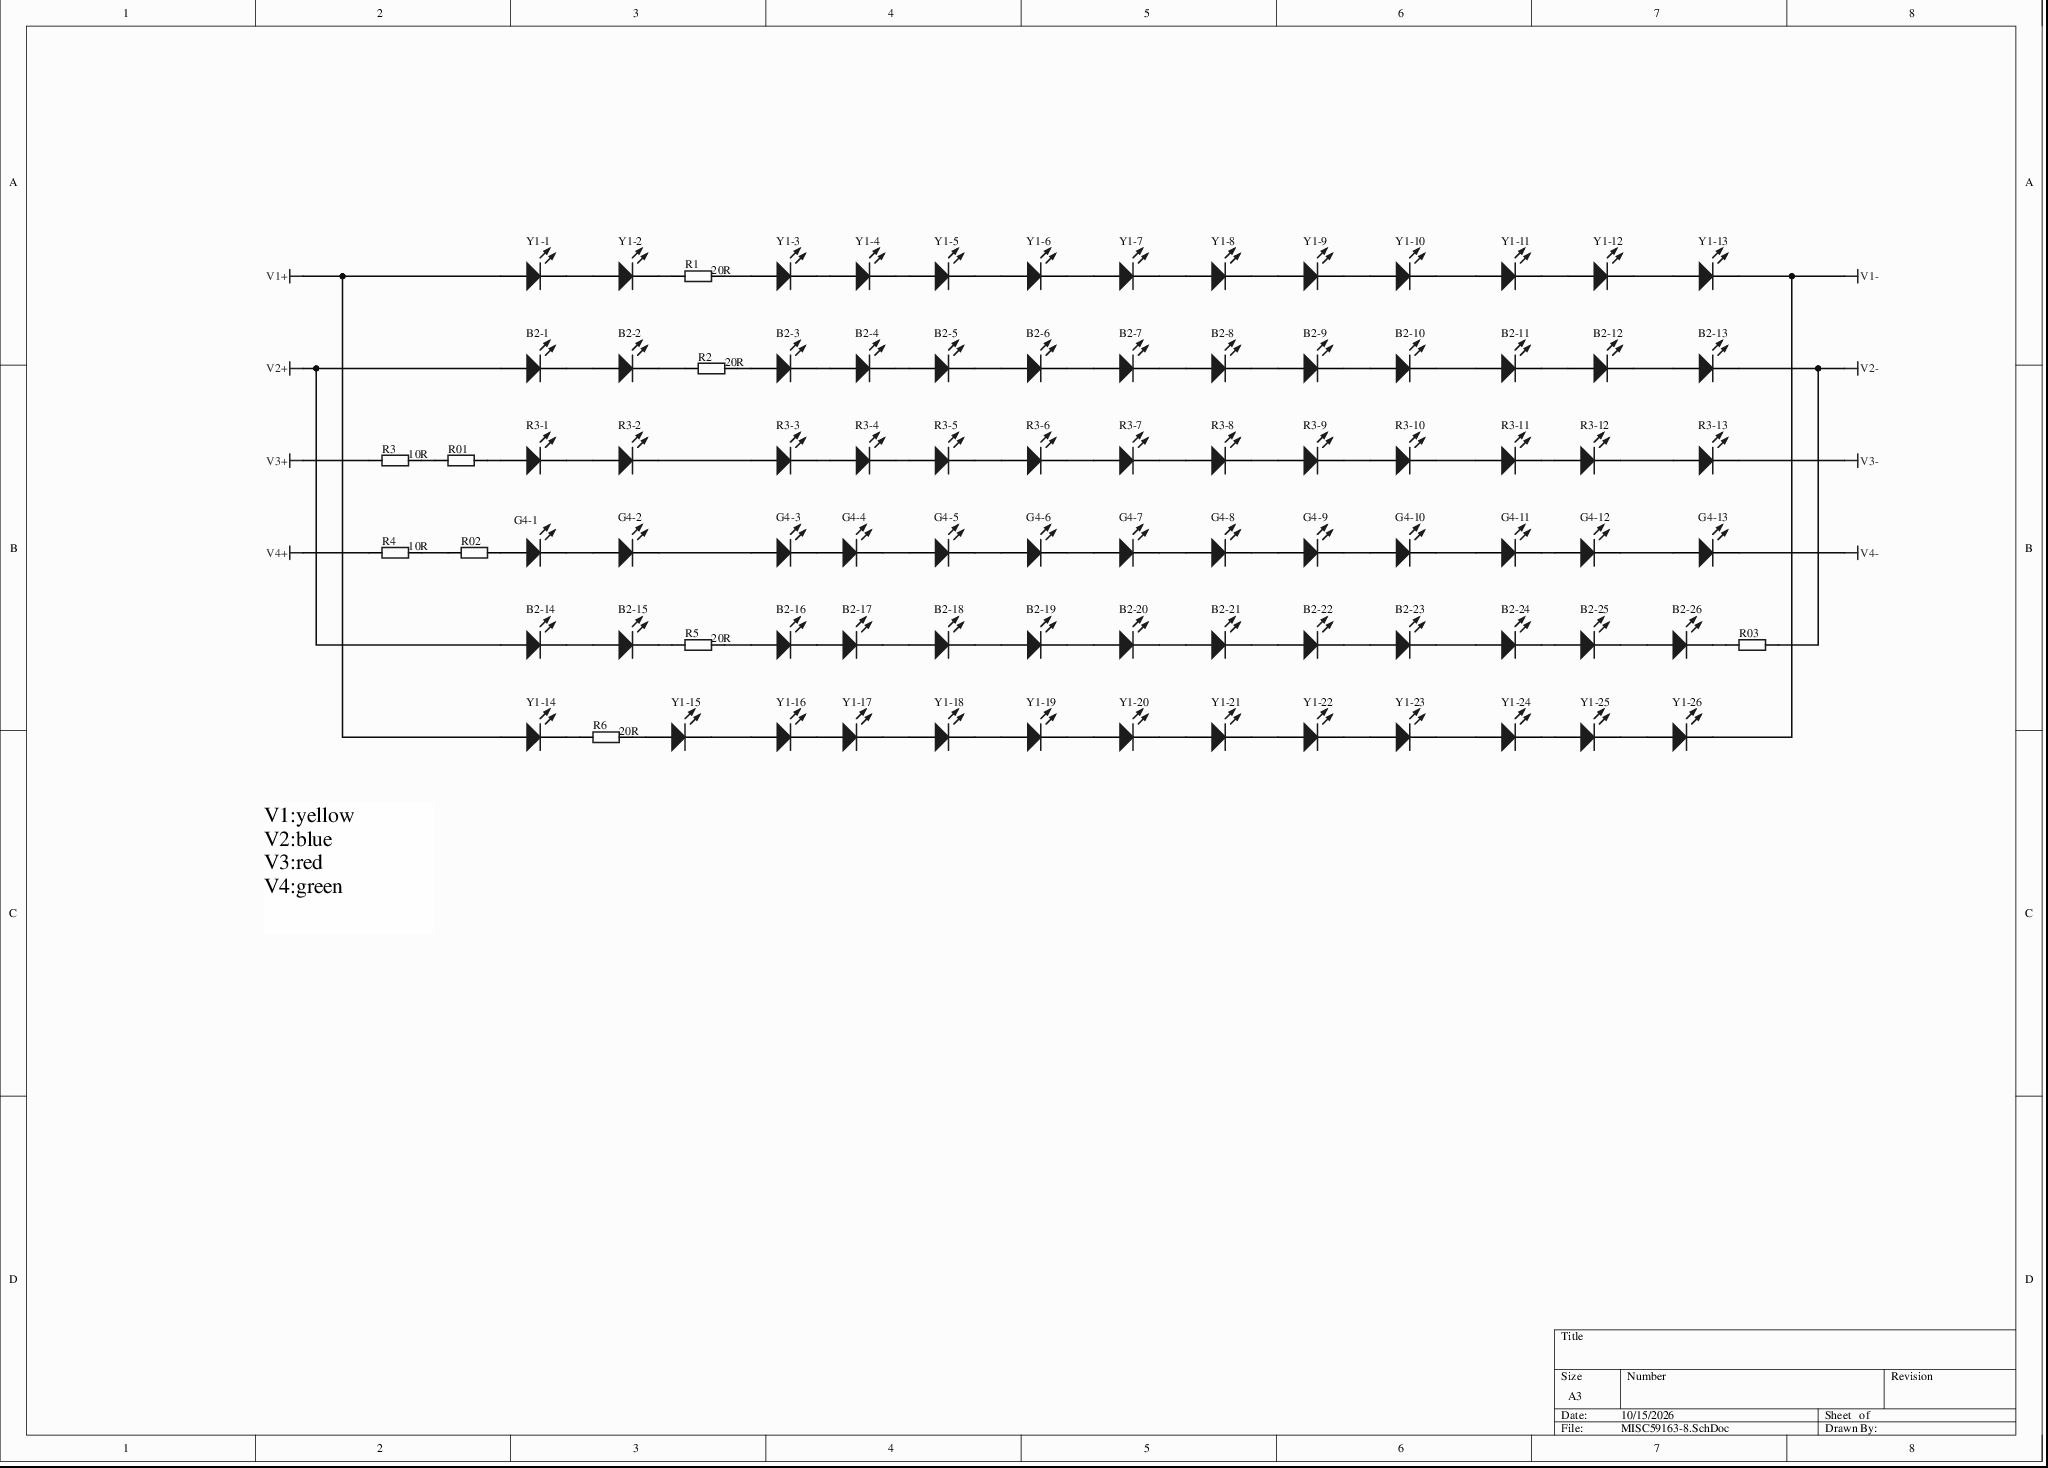
[diagram p0: MISC59163-8.SchDoc]
# Altium project MISC59163-2.PrjPcb
1 sheet, 87 parts. Net scope: global (net labels, ports and power ports of the same name join across sheets).
Board file: MISC59163.PcbDoc

## Sheet MISC59163-8.SchDoc
size A3; SheetNumber: 1; SheetTotal: 1

### Parts
B2-1  2835A03-480B05-1S-F8  [2835LED带透镜]  (value not drawn)
B2-2  2835A03-480B05-1S-F8  [2835LED带透镜]  (value not drawn)
B2-3  2835A03-480B05-1S-F8  [2835LED带透镜]  (value not drawn)
B2-4  2835A03-480B05-1S-F8  [2835LED带透镜]  (value not drawn)
B2-5  2835A03-480B05-1S-F8  [2835LED带透镜]  (value not drawn)
B2-6  2835A03-480B05-1S-F8  [2835LED带透镜]  (value not drawn)
B2-7  2835A03-480B05-1S-F8  [2835LED带透镜]  (value not drawn)
B2-8  2835A03-480B05-1S-F8  [2835LED带透镜]  (value not drawn)
B2-9  2835A03-480B05-1S-F8  [2835LED带透镜]  (value not drawn)
B2-10  2835A03-480B05-1S-F8  [2835LED带透镜]  (value not drawn)
B2-11  2835A03-480B05-1S-F8  [2835LED带透镜]  (value not drawn)
B2-12  2835A03-480B05-1S-F8  [2835LED带透镜]  (value not drawn)
B2-13  2835A03-480B05-1S-F8  [2835LED带透镜]  (value not drawn)
B2-14  2835A03-480B05-1S-F8  [2835LED带透镜2]  (value not drawn)
B2-15  2835A03-480B05-1S-F8  [2835LED带透镜2]  (value not drawn)
B2-16  2835A03-480B05-1S-F8  [2835LED带透镜2]  (value not drawn)
B2-17  2835A03-480B05-1S-F8  [2835LED带透镜2]  (value not drawn)
B2-18  2835A03-480B05-1S-F8  [2835LED带透镜2]  (value not drawn)
B2-19  2835A03-480B05-1S-F8  [2835LED带透镜2]  (value not drawn)
B2-20  2835A03-480B05-1S-F8  [2835LED带透镜2]  (value not drawn)
B2-21  2835A03-480B05-1S-F8  [2835LED带透镜2]  (value not drawn)
B2-22  2835A03-480B05-1S-F8  [2835LED带透镜2]  (value not drawn)
B2-23  2835A03-480B05-1S-F8  [2835LED带透镜2]  (value not drawn)
B2-24  2835A03-480B05-1S-F8  [2835LED带透镜2]  (value not drawn)
B2-25  2835A03-480B05-1S-F8  [2835LED带透镜2]  (value not drawn)
B2-26  2835A03-480B05-1S-F8  [2835LED带透镜2]  (value not drawn)
G4-1  2835A03-525G05-2P-F10  [2835LED带透镜3]  (value not drawn)
G4-2  2835A03-525G05-2P-F10  [2835LED带透镜3]  (value not drawn)
G4-3  2835A03-525G05-2P-F10  [2835LED带透镜3]  (value not drawn)
G4-4  2835A03-525G05-2P-F10  [2835LED带透镜3]  (value not drawn)
G4-5  2835A03-525G05-2P-F10  [2835LED带透镜3]  (value not drawn)
G4-6  2835A03-525G05-2P-F10  [2835LED带透镜3]  (value not drawn)
G4-7  2835A03-525G05-2P-F10  [2835LED带透镜3]  (value not drawn)
G4-8  2835A03-525G05-2P-F10  [2835LED带透镜3]  (value not drawn)
G4-9  2835A03-525G05-2P-F10  [2835LED带透镜3]  (value not drawn)
G4-10  2835A03-525G05-2P-F10  [2835LED带透镜3]  (value not drawn)
G4-11  2835A03-525G05-2P-F10  [2835LED带透镜3]  (value not drawn)
G4-12  2835A03-525G05-2P-F10  [2835LED带透镜3]  (value not drawn)
G4-13  2835A03-525G05-2P-F10  [2835LED带透镜2]  (value not drawn)
R1  value 20R  [R0805]  (hidden comment: 20Ω)
R01  jumper  [贴片跳线QM8.2-D01]  (value not drawn)
R2  value 20R  [R0805]  (hidden comment: 20Ω)
R02  jumper  [贴片跳线QM8.2-D01]  (value not drawn)
R3  value 10R  [R0805]  (hidden comment: 10Ω)
R03  jumper  [贴片跳线]  (value not drawn)
R3-1  2835A03-630R05-2P-F10  [2835LED带透镜3]  (value not drawn)
R3-2  2835A03-630R05-2P-F10  [2835LED带透镜3]  (value not drawn)
R3-3  2835A03-630R05-2P-F10  [2835LED带透镜3]  (value not drawn)
R3-4  2835A03-630R05-2P-F10  [2835LED带透镜3]  (value not drawn)
R3-5  2835A03-630R05-2P-F10  [2835LED带透镜3]  (value not drawn)
R3-6  2835A03-630R05-2P-F10  [2835LED带透镜3]  (value not drawn)
R3-7  2835A03-630R05-2P-F10  [2835LED带透镜3]  (value not drawn)
R3-8  2835A03-630R05-2P-F10  [2835LED带透镜3]  (value not drawn)
R3-9  2835A03-630R05-2P-F10  [2835LED带透镜3]  (value not drawn)
R3-10  2835A03-630R05-2P-F10  [2835LED带透镜3]  (value not drawn)
R3-11  2835A03-630R05-2P-F10  [2835LED带透镜3]  (value not drawn)
R3-12  2835A03-630R05-2P-F10  [2835LED带透镜3]  (value not drawn)
R3-13  2835A03-630R05-2P-F10  [2835LED带透镜3]  (value not drawn)
R4  value 10R  [R0805]  (hidden comment: 10Ω)
R5  value 20R  [R0805]  (hidden comment: 20Ω)
R6  value 20R  [R0805]  (hidden comment: 20Ω)
Y1-1  2835A03-585Y05-2P-F10  [2835LED带透镜1]  (value not drawn)
Y1-2  2835A03-585Y05-2P-F10  [2835LED带透镜]  (value not drawn)
Y1-3  2835A03-585Y05-2P-F10  [2835LED带透镜]  (value not drawn)
Y1-4  2835A03-585Y05-2P-F10  [2835LED带透镜]  (value not drawn)
Y1-5  2835A03-585Y05-2P-F10  [2835LED带透镜]  (value not drawn)
Y1-6  2835A03-585Y05-2P-F10  [2835LED带透镜]  (value not drawn)
Y1-7  2835A03-585Y05-2P-F10  [2835LED带透镜]  (value not drawn)
Y1-8  2835A03-585Y05-2P-F10  [2835LED带透镜]  (value not drawn)
Y1-9  2835A03-585Y05-2P-F10  [2835LED带透镜]  (value not drawn)
Y1-10  2835A03-585Y05-2P-F10  [2835LED带透镜]  (value not drawn)
Y1-11  2835A03-585Y05-2P-F10  [2835LED带透镜]  (value not drawn)
Y1-12  2835A03-585Y05-2P-F10  [2835LED带透镜]  (value not drawn)
Y1-13  2835A03-585Y05-2P-F10  [2835LED带透镜]  (value not drawn)
Y1-14  2835A03-585Y05-2P-F10  [2835LED带透镜2]  (value not drawn)
Y1-15  2835A03-585Y05-2P-F10  [2835LED带透镜2]  (value not drawn)
Y1-16  2835A03-585Y05-2P-F10  [2835LED带透镜2]  (value not drawn)
Y1-17  2835A03-585Y05-2P-F10  [2835LED带透镜2]  (value not drawn)
Y1-18  2835A03-585Y05-2P-F10  [2835LED带透镜2]  (value not drawn)
Y1-19  2835A03-585Y05-2P-F10  [2835LED带透镜2]  (value not drawn)
Y1-20  2835A03-585Y05-2P-F10  [2835LED带透镜2]  (value not drawn)
Y1-21  2835A03-585Y05-2P-F10  [2835LED带透镜2]  (value not drawn)
Y1-22  2835A03-585Y05-2P-F10  [2835LED带透镜2]  (value not drawn)
Y1-23  2835A03-585Y05-2P-F10  [2835LED带透镜2]  (value not drawn)
Y1-24  2835A03-585Y05-2P-F10  [2835LED带透镜2]  (value not drawn)
Y1-25  2835A03-585Y05-2P-F10  [2835LED带透镜2]  (value not drawn)
Y1-26  2835A03-585Y05-2P-F10  [2835LED带透镜2]  (value not drawn)

### Nets
V1+: Y1-1.1(A) Y1-14.1(A)
V1-: Y1-13.2(K) Y1-26.2(K)
V2+: B2-1.1(A) B2-14.1(A)
V2-: B2-13.2(K) R03.2
V3+: R3.1
V3-: R3-13.1(K)
V4+: R4.1
V4-: G4-13.2(K)
NetB2-1_2: B2-1.2(K) B2-2.1(A)
NetB2-2_2: B2-2.2(K) R2.1
NetB2-3_1: B2-3.1(A) R2.2
NetB2-3_2: B2-3.2(K) B2-4.1(A)
NetB2-4_2: B2-4.2(K) B2-5.1(A)
NetB2-5_2: B2-5.2(K) B2-6.1(A)
NetB2-6_2: B2-6.2(K) B2-7.1(A)
NetB2-7_2: B2-7.2(K) B2-8.1(A)
NetB2-8_2: B2-8.2(K) B2-9.1(A)
NetB2-9_2: B2-9.2(K) B2-10.1(A)
NetB2-10_2: B2-10.2(K) B2-11.1(A)
NetB2-11_2: B2-11.2(K) B2-12.1(A)
NetB2-12_2: B2-12.2(K) B2-13.1(A)
NetB2-14_2: B2-14.2(K) B2-15.1(A)
NetB2-15_2: B2-15.2(K) R5.1
NetB2-16_1: B2-16.1(A) R5.2
NetB2-16_2: B2-16.2(K) B2-17.1(A)
NetB2-17_2: B2-17.2(K) B2-18.1(A)
NetB2-18_2: B2-18.2(K) B2-19.1(A)
NetB2-19_2: B2-19.2(K) B2-20.1(A)
NetB2-20_2: B2-20.2(K) B2-21.1(A)
NetB2-21_2: B2-21.2(K) B2-22.1(A)
NetB2-22_2: B2-22.2(K) B2-23.1(A)
NetB2-23_2: B2-23.2(K) B2-24.1(A)
NetB2-24_2: B2-24.2(K) B2-25.1(A)
NetB2-25_2: B2-25.2(K) B2-26.1(A)
NetB2-26_2: B2-26.2(K) R03.1
NetG4-1_1: G4-1.1(A) R02.2
NetG4-1_2: G4-1.2(K) G4-2.1(A)
NetG4-2_2: G4-2.2(K) G4-3.1(A)
NetG4-3_2: G4-3.2(K) G4-4.1(A)
NetG4-4_2: G4-4.2(K) G4-5.1(A)
NetG4-5_2: G4-5.2(K) G4-6.1(A)
NetG4-6_2: G4-6.2(K) G4-7.1(A)
NetG4-7_2: G4-7.2(K) G4-8.1(A)
NetG4-8_2: G4-8.2(K) G4-9.1(A)
NetG4-9_2: G4-9.2(K) G4-10.1(A)
NetG4-10_2: G4-10.2(K) G4-11.1(A)
NetG4-11_2: G4-11.2(K) G4-12.1(A)
NetG4-12_2: G4-12.2(K) G4-13.1(A)
NetR1_1: R1.1 Y1-2.2(K)
NetR01_1: R01.1 R3.2
NetR1_2: R1.2 Y1-3.1(A)
NetR01_2: R01.2 R3-1.2(A)
NetR02_1: R02.1 R4.2
NetR3-1_1: R3-1.1(K) R3-2.2(A)
NetR3-2_1: R3-2.1(K) R3-3.2(A)
NetR3-3_1: R3-3.1(K) R3-4.2(A)
NetR3-4_1: R3-4.1(K) R3-5.2(A)
NetR3-5_1: R3-5.1(K) R3-6.2(A)
NetR3-6_1: R3-6.1(K) R3-7.2(A)
NetR3-7_1: R3-7.1(K) R3-8.2(A)
NetR3-8_1: R3-8.1(K) R3-9.2(A)
NetR3-9_1: R3-9.1(K) R3-10.2(A)
NetR3-10_1: R3-10.1(K) R3-11.2(A)
NetR3-11_1: R3-11.1(K) R3-12.2(A)
NetR3-12_1: R3-12.1(K) R3-13.2(A)
NetR6_1: R6.1 Y1-14.2(K)
NetR6_2: R6.2 Y1-15.1(A)
NetY1-1_2: Y1-1.2(K) Y1-2.1(A)
NetY1-3_2: Y1-3.2(K) Y1-4.1(A)
NetY1-4_2: Y1-4.2(K) Y1-5.1(A)
NetY1-5_2: Y1-5.2(K) Y1-6.1(A)
NetY1-6_2: Y1-6.2(K) Y1-7.1(A)
NetY1-7_2: Y1-7.2(K) Y1-8.1(A)
NetY1-8_2: Y1-8.2(K) Y1-9.1(A)
NetY1-9_2: Y1-9.2(K) Y1-10.1(A)
NetY1-10_2: Y1-10.2(K) Y1-11.1(A)
NetY1-11_2: Y1-11.2(K) Y1-12.1(A)
NetY1-12_2: Y1-12.2(K) Y1-13.1(A)
NetY1-15_2: Y1-15.2(K) Y1-16.1(A)
NetY1-16_2: Y1-16.2(K) Y1-17.1(A)
NetY1-17_2: Y1-17.2(K) Y1-18.1(A)
NetY1-18_2: Y1-18.2(K) Y1-19.1(A)
NetY1-19_2: Y1-19.2(K) Y1-20.1(A)
NetY1-20_2: Y1-20.2(K) Y1-21.1(A)
NetY1-21_2: Y1-21.2(K) Y1-22.1(A)
NetY1-22_2: Y1-22.2(K) Y1-23.1(A)
NetY1-23_2: Y1-23.2(K) Y1-24.1(A)
NetY1-24_2: Y1-24.2(K) Y1-25.1(A)
NetY1-25_2: Y1-25.2(K) Y1-26.1(A)

### Notes on the sheet
- V1:yellow
  V2:blue
  V3:red
  V4:green

### Library data of the parts
B2-1-B2-26 G4-1-G4-13 R3-1-R3-13 Y1-1-Y1-26 = LED2: Published: 8-Jun-2000; LatestRevisionDate: 17-Jul-2002; LatestRevisionNote: Re-released for DXP Platform.; PackageVersion: Feb-2002; PackageReference: 3.2X1.6X1.1; PackageDescription: SM LED; 2 Flat Leads; Publisher: Altium Limited
R1-R6 = Res2: 0805 chip resistor; Published: 8-Jun-2000; LatestRevisionDate: 17-Jul-2002; LatestRevisionNote: Re-released for DXP Platform.; PackageReference: AXIAL-0.4; PackageDescription: Axial Device, Thru-Hole; 2 Leads; 0.4 in Pin Spacing; Publisher: Altium Limited
R01 R02 = Res2: QM8.2-D01  silver; Published: 8-Jun-2000; LatestRevisionDate: 17-Jul-2002; LatestRevisionNote: Re-released for DXP Platform.; PackageReference: AXIAL-0.4; PackageDescription: Axial Device, Thru-Hole; 2 Leads; 0.4 in Pin Spacing; Publisher: Altium Limited
R03 = Res2: QM52-D01  silver; Published: 8-Jun-2000; LatestRevisionDate: 17-Jul-2002; LatestRevisionNote: Re-released for DXP Platform.; PackageReference: AXIAL-0.4; PackageDescription: Axial Device, Thru-Hole; 2 Leads; 0.4 in Pin Spacing; Publisher: Altium Limited